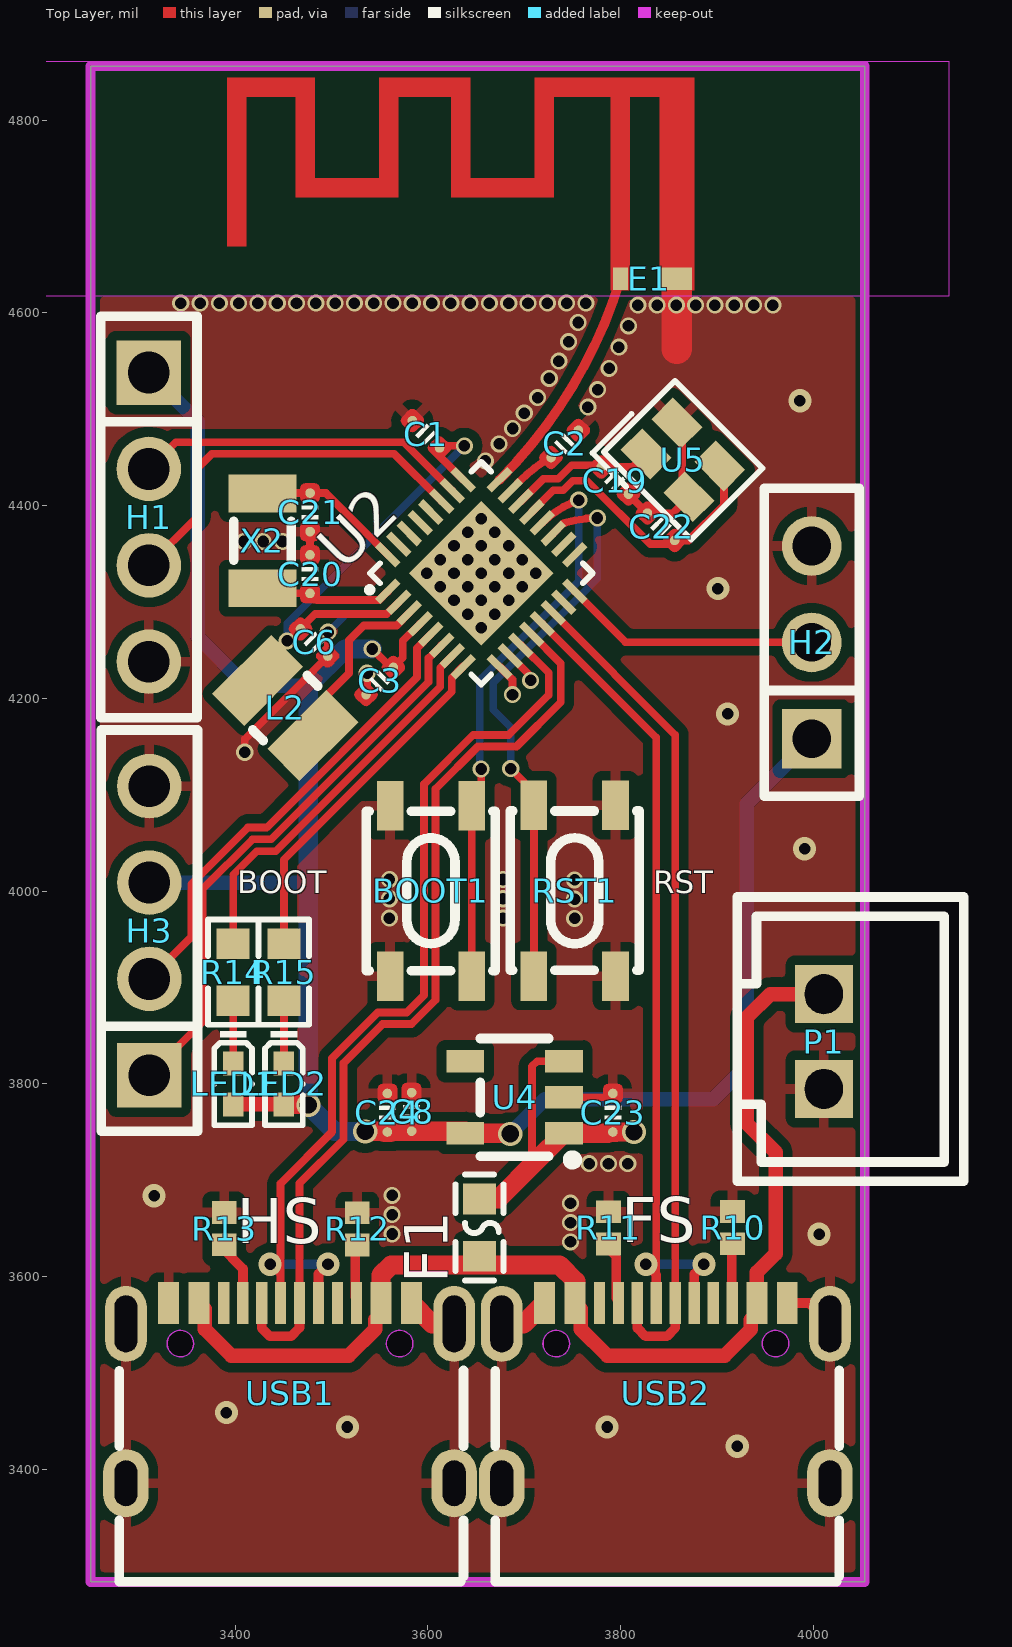
[diagram p0: Top Layer view]
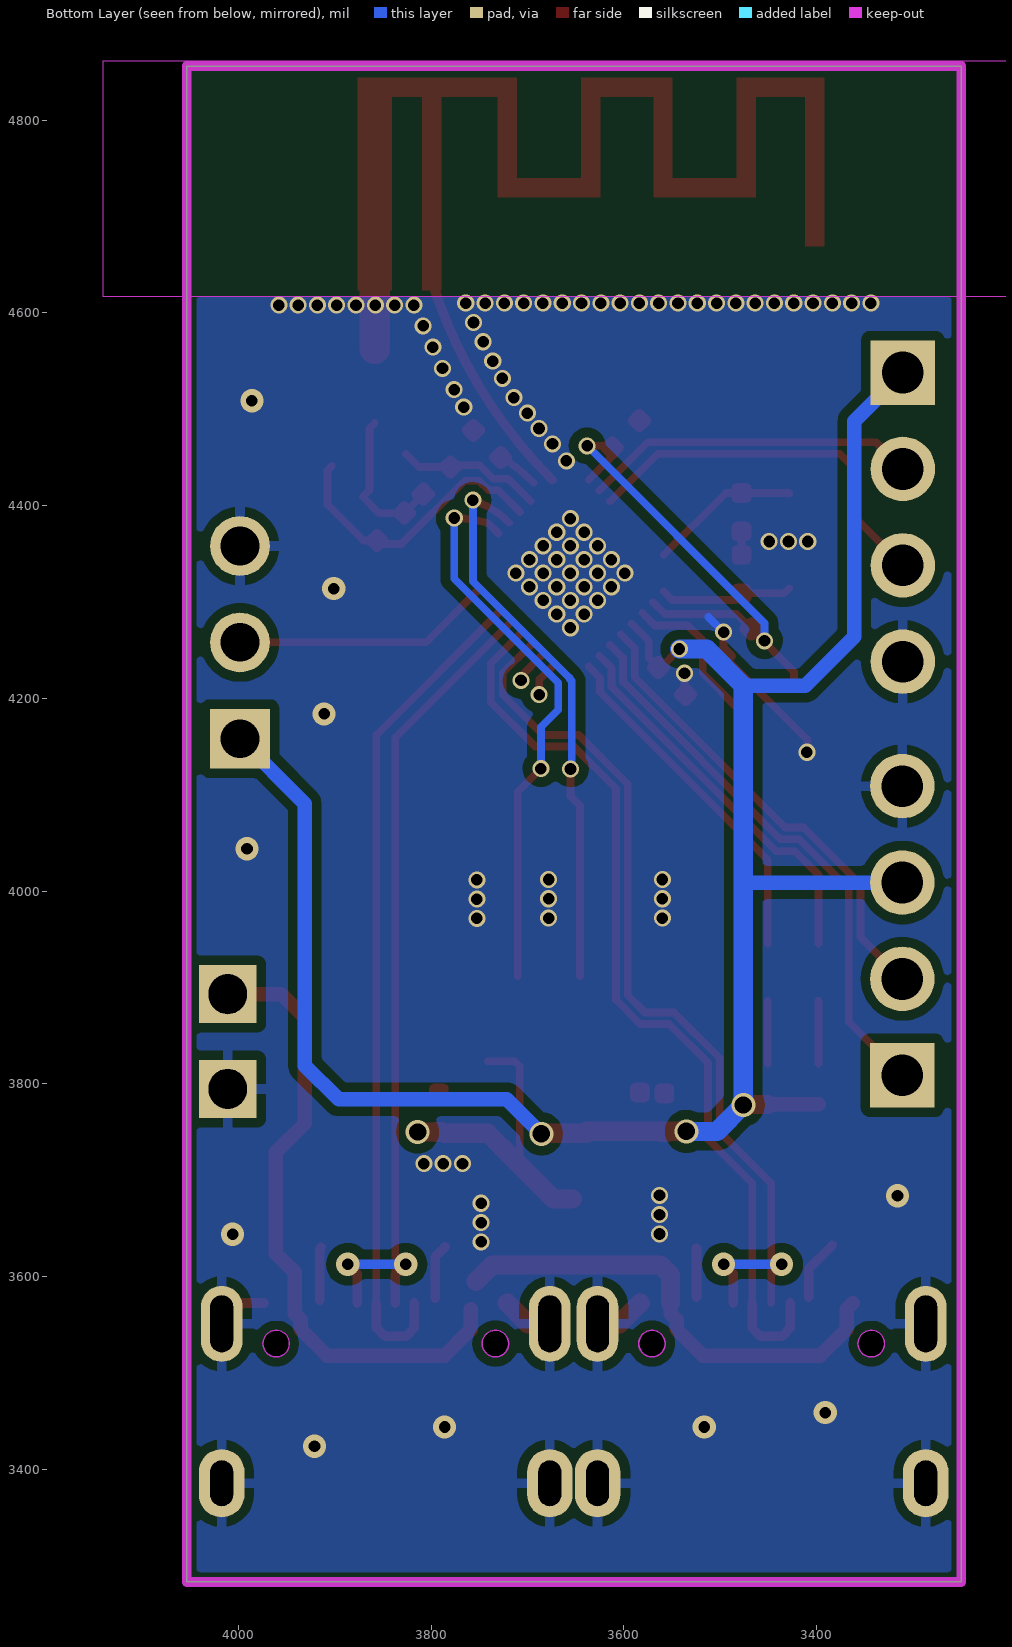
[diagram p1: Bottom Layer view, seen from below]
# Altium PCB MISC75430.pcbdoc
Units mil, origin at the board's own origin, x right, y up, seen from the top; angles counter-clockwise.
Board outline 803.38 x 1573.11 mil, 2 copper layers (Top Layer, Bottom Layer), stack 62.206 mil thick; 34 components, 40 nets, 141 pads, 120 vias.

## Layer stack, top to bottom
Top Solder Mask Layer: solder mask 0.394, Dk 3.3
Top Layer: signal copper 1.379
SUBSTRATE1: surface 59.449, FR4, Dk 4.5
Bottom Layer: signal copper 1.378
Bottom Solder Mask Layer: solder mask 0.394, Dk 3.3

## Board outline
3250,4856.14 3250,3283.03 4053.38,3283.03 4053.38,4856.14

## Design rules (kind name [scope] priority, off if disabled: settings)
BoardOutlineClearance copperThickness2oz_1 [All] p2 off: genericclearance=7.99 ignorepadtopadclearanceinfootprint=FALSE except(0: Arc-SplitContinuation Track-SplitContinuation SMDPad-SplitContinuation THPad-SplitContinuation Via-SplitContinuation Fill-SplitContinuation Region-SplitContinuation Poly-SplitContinuation Text-SplitContinuation Hole-SplitContinuation; 5.98: Arc-CutoutEdge Track-CutoutEdge SMDPad-CutoutEdge THPad-CutoutEdge Via-CutoutEdge Text-CutoutEdge; 6.9: Hole-OutlineEdge Hole-CutoutEdge; 10: Poly-OutlineEdge Poly-CutoutEdge; 11.81: Arc-OutlineEdge Track-OutlineEdge SMDPad-OutlineEdge THPad-OutlineEdge Via-OutlineEdge Fill-OutlineEdge Region-OutlineEdge Text-OutlineEdge Fill-CutoutEdge Region-CutoutEdge)
BoardOutlineClearance Plane_innerPlane_1 [All] p4 off: genericclearance=4.02 ignorepadtopadclearanceinfootprint=FALSE except(0: Arc-SplitContinuation Track-SplitContinuation SMDPad-SplitContinuation THPad-SplitContinuation Via-SplitContinuation Fill-SplitContinuation Region-SplitContinuation Poly-SplitContinuation Text-SplitContinuation Hole-SplitContinuation; 5.98: Arc-CutoutEdge Track-CutoutEdge SMDPad-CutoutEdge THPad-CutoutEdge Via-CutoutEdge Text-CutoutEdge; 6.9: Hole-OutlineEdge Hole-CutoutEdge; 10: Poly-OutlineEdge Poly-CutoutEdge; 11.81: Arc-OutlineEdge Track-OutlineEdge SMDPad-OutlineEdge THPad-OutlineEdge Via-OutlineEdge Fill-OutlineEdge Region-OutlineEdge Text-OutlineEdge Fill-CutoutEdge Region-CutoutEdge)
BoardOutlineClearance Copper_copperRegion_1 [All] p6 off: genericclearance=4.02 ignorepadtopadclearanceinfootprint=FALSE except(0: Arc-SplitContinuation Track-SplitContinuation SMDPad-SplitContinuation THPad-SplitContinuation Via-SplitContinuation Fill-SplitContinuation Region-SplitContinuation Poly-SplitContinuation Text-SplitContinuation Hole-SplitContinuation; 5.98: Arc-CutoutEdge Track-CutoutEdge SMDPad-CutoutEdge THPad-CutoutEdge Via-CutoutEdge Text-CutoutEdge; 6.9: Hole-OutlineEdge Hole-CutoutEdge; 10: Poly-OutlineEdge Poly-CutoutEdge; 11.81: Arc-OutlineEdge Track-OutlineEdge SMDPad-OutlineEdge THPad-OutlineEdge Via-OutlineEdge Fill-OutlineEdge Region-OutlineEdge Text-OutlineEdge Fill-CutoutEdge Region-CutoutEdge)
BoardOutlineClearance copperThickness1oz_1 [All] p8: genericclearance=0 ignorepadtopadclearanceinfootprint=FALSE except(0: Arc-OutlineEdge Track-OutlineEdge SMDPad-OutlineEdge THPad-OutlineEdge Via-OutlineEdge Fill-OutlineEdge Region-OutlineEdge Poly-OutlineEdge Text-OutlineEdge Hole-OutlineEdge Arc-CutoutEdge Track-CutoutEdge SMDPad-CutoutEdge THPad-CutoutEdge Via-CutoutEdge Fill-CutoutEdge Region-CutoutEdge Poly-CutoutEdge Text-CutoutEdge Hole-CutoutEdge Arc-SplitContinuation Track-SplitContinuation SMDPad-SplitContinuation THPad-SplitContinuation Via-SplitContinuation Fill-SplitContinuation Region-SplitContinuation Poly-SplitContinuation Text-SplitContinuation Hole-SplitContinuation)
Clearance copperThickness2oz [All] p1 off: gap=7.99 ignorepadtopadclearanceinfootprint=FALSE except(5.98: SMDPad-Track SMDPad-SMDPad THPad-Track SMDPad-THPad THPad-THPad Track-Via SMDPad-Via THPad-Via Via-Via Fill-SMDPad Region-SMDPad Fill-THPad Region-THPad Fill-Via Region-Via Fill-Fill Fill-Region Region-Region Arc-Track Arc-SMDPad Arc-THPad Arc-Via Fill-Arc Region-Arc Arc-Arc Text-Track SMDPad-Text Text-THPad Text-Via Fill-Text Region-Text Arc-Text Text-Text; 6.9: Hole-Track Hole-SMDPad Hole-THPad Hole-Via Fill-Hole Region-Hole Hole-Arc Hole-Text; 10: Poly-Track Poly-SMDPad Poly-THPad Poly-Via Poly-Fill Poly-Region Poly-Poly Poly-Arc Poly-Text Poly-Hole; 11.81: Fill-Track Region-Track)
Clearance Plane_innerPlane [All] p3 off: gap=4.02 ignorepadtopadclearanceinfootprint=FALSE except(5.98: SMDPad-Track SMDPad-SMDPad THPad-Track SMDPad-THPad THPad-THPad Track-Via SMDPad-Via THPad-Via Via-Via Fill-SMDPad Region-SMDPad Fill-THPad Region-THPad Fill-Via Region-Via Fill-Fill Fill-Region Region-Region Arc-Track Arc-SMDPad Arc-THPad Arc-Via Fill-Arc Region-Arc Arc-Arc Text-Track SMDPad-Text Text-THPad Text-Via Fill-Text Region-Text Arc-Text Text-Text; 6.9: Hole-Track Hole-SMDPad Hole-THPad Hole-Via Fill-Hole Region-Hole Hole-Arc Hole-Text; 10: Poly-Track Poly-SMDPad Poly-THPad Poly-Via Poly-Fill Poly-Region Poly-Poly Poly-Arc Poly-Text Poly-Hole; 11.81: Fill-Track Region-Track)
Clearance Copper_copperRegion [All] p5 off: gap=4.02 ignorepadtopadclearanceinfootprint=FALSE except(5.98: SMDPad-Track SMDPad-SMDPad THPad-Track SMDPad-THPad THPad-THPad Track-Via SMDPad-Via THPad-Via Via-Via Fill-SMDPad Region-SMDPad Fill-THPad Region-THPad Fill-Via Region-Via Fill-Fill Fill-Region Region-Region Arc-Track Arc-SMDPad Arc-THPad Arc-Via Fill-Arc Region-Arc Arc-Arc Text-Track SMDPad-Text Text-THPad Text-Via Fill-Text Region-Text Arc-Text Text-Text; 6.9: Hole-Track Hole-SMDPad Hole-THPad Hole-Via Fill-Hole Region-Hole Hole-Arc Hole-Text; 10: Poly-Track Poly-SMDPad Poly-THPad Poly-Via Poly-Fill Poly-Region Poly-Poly Poly-Arc Poly-Text Poly-Hole; 11.81: Fill-Track Region-Track)
Clearance copperThickness1oz [All] p7: gap=0 ignorepadtopadclearanceinfootprint=FALSE
DiffPairsRouting differentialPair [All] p1: maxlimit=6 minlimit=6 mostfreqgap=6 toplayer_minwidth=5 toplayer_prefwidth=10 toplayer_maxwidth=100 toplayer_mingap=6 toplayer_prefgap=6 toplayer_maxgap=6 bottomlayer_minwidth=5 bottomlayer_prefwidth=10 bottomlayer_maxwidth=100 bottomlayer_mingap=6 bottomlayer_prefgap=6 bottomlayer_maxgap=6 maxuncoupledlength=10
HoleToHoleClearance otherClearance [All] p1: gap=0 allowstackedmicrovias=TRUE
Length netLength [All] p1: minlimit=0 maxlimit=0
MatchedLengths netLengthTolerance [All] p1: tolerance=1000
PasteMaskExpansion pasteMaskExpansion [All] p1: expansion=0
PlaneConnect innerPlane [All] p1: planeconnectstyle=Relief reliefexpansion=20 reliefentries=4 reliefconductorwidth=10 reliefairgap=10
PolygonConnect copperRegion [All] p1: connectstyle=Relief reliefconductorwidth=10 reliefentries=4 polygonreliefangle="90 Angle" airgapwidth=10 via.connectstyle=Relief via.reliefconductorwidth=10 via.reliefentries=4 via.polygonreliefangle="90 Angle" via.airgapwidth=10
RoutingVias viaSize [All] p1: holewidth=0.39 width=0.39 viastyle="Through Hole" minholewidth=0.39 minwidth=0.39 maxholewidth=472.44 maxwidth=472.44
SolderMaskExpansion solderMaskExpansion [IsVia] p1: expansion=-1000 istentingtop=TRUE
SolderMaskExpansion solderMaskExpansion [All] p2: expansion=2 istentingtop=FALSE
Width copperThickness2oz_2 [All] p1 off: maxlimit=10 minlimit=10 preferedwidth=10 toplayer_minwidth=8 toplayer_maxwidth=100 toplayer_prefwidth=10 bottomlayer_minwidth=8 bottomlayer_maxwidth=100 bottomlayer_prefwidth=10
Width copperThickness1oz_2 [All] p2: maxlimit=10 minlimit=10 preferedwidth=10 toplayer_minwidth=5 toplayer_maxwidth=100 toplayer_prefwidth=10 bottomlayer_minwidth=5 bottomlayer_maxwidth=100 bottomlayer_prefwidth=10

## Components (designator, comment, footprint, x,y, rotation, side; value= is the part's Value field where it differs from the comment)
BOOT1 "K2-1808SN-A3SW-01" SW-SMD_4P-L4.2-W3.3-P2.15-LS5.1 3603.12,4000.1 r270 top
C1 "100nF" 0402电容（极简封装） 3598,4474 r135 top
C2 "470nF" 0402电容（极简封装） 3742,4464 r45 top
C3 "2.2uF" 0402电容（极简封装） 3550,4218 r225 top
C6 "4.7uF" 0402电容（极简封装） 3482,4258 r135 top
C8 "100nF" 0402电容（极简封装） 3583.17,3770.84 r270 top
C19 "NC" 0402电容（极简封装） 3794,4426 r135 top
C20 "NC" 0402电容（极简封装） 3477.72,4328.89 r90 top
C21 "NC" 0402电容（极简封装） 3477.81,4392.99 r270 top
C22 "NC" 0402电容（极简封装） 3842,4378 r315 top
C23 "1uF" 0402电容（极简封装） 3792,3770 r270 top
C24 "1uF" 0402电容（极简封装） 3558,3770 r270 top
E1 "" ANT-F-1-2.4G-1.6mmFR4 3662.08,4744.9 r0 top
F1 "BSMD0603-050-6V" F0603 3653.63,3650.83 r90 top
H1 "" HDR-TH_4P-P2.54-V-F 3310.5,4388.05 r270 top
H2 "" HDR-TH_3P-P2.54-V-F 3998.3,4258.05 r90 top
H3 "" HDR-TH_4P-P2.54-V-F 3311,3958.85 r90 top
L2 "10uH" IND-SMD_L2.5-W2.0 3452,4190 r135 top
LED1 "SZYY0402B" LED0402-RD_BLUE 3397.95,3799.79 r270 top
LED2 "SZYY0402B" LED0402-RD_BLUE 3450.63,3799.79 r270 top
P1 "XH2.54 through-hole socket-2P" CONN-TH_XH2.54-2P 4011,3843.85 r270 top
R10 "5.1kΩ" R0402 3916.19,3650.84 r270 top
R11 "5.1kΩ" R0402 3787.44,3650.56 r270 top
R12 "5.1kΩ" R0402 3526.84,3649.44 r270 top
R13 "5.1kΩ" R0402 3388.65,3649.68 r270 top
R14 "1kΩ" R0603 3397.95,3915.83 r270 top
R15 "1kΩ" R0603 3450.63,3915.83 r270 top
RST1 "K2-1808SN-A3SW-01" SW-SMD_4P-L4.2-W3.3-P2.15-LS5.1 3752.41,4000.34 r90 top
U2 "CH584F" QFN-32_L4.0-W4.0-P0.40-TL-EP2.7 3655.44,4329.85 r45 top
U4 "RT9013-33GB" SOT-23-5_L3.0-W1.7-P0.95-LS2.8-BR 3690,3786 r0 top
U5 "32MHz" CRYSTAL-SMD_4P-L2.0-W1.6-BL-2 3864.68,4447.36 r315 top
USB1 "TYPE-C 16PIN 2MD(073)" USB-C-SMD_TYPE-C-6PIN-2MD-073 3457,3479 r0 top
USB2 "TYPE-C 16PIN 2MD(073)" USB-C-SMD_TYPE-C-6PIN-2MD-073 3847,3479 r0 top
X2 "32.768kHz" FC-135R_L3.2-W1.5 3428.4,4363.43 r90 top

## Footprints (in the part's own frame and the unit in brackets; to place one, negate y for a bottom-side part, rotate by r counter-clockwise, add the part's x,y. Pads: shape width x height; smd on the part's side, far side on the other; paste and mask are expansions set on the pad)
0402电容（极简封装） [mil]
  round 10 smd: 1(-20,0) 2(20,0)
  Top Layer region: 30,-5 29.62,-6.91 28.54,-8.54 26.91,-9.62 25,-10 15,-10 13.09,-9.62 11.46,-8.54 10.38,-6.91 10,-5 10,5 10.38,6.91 11.46,8.54 13.09,9.62 15,10 25,10 26.91,9.62 28.54,8.54 29.62,6.91 30,5 30,-5
  Top Layer region: -10,-5 -10.38,-6.91 -11.46,-8.54 -13.09,-9.62 -15,-10 -25,-10 -26.91,-9.62 -28.54,-8.54 -29.62,-6.91 -30,-5 -30,5 -29.62,6.91 -28.54,8.54 -26.91,9.62 -25,10 -15,10 -13.09,9.62 -11.46,8.54 -10.38,6.91 -10,5 -10,-5
  silkscreen extent -7,-9 7,9
ANT-F-1-2.4G-1.6mmFR4 [mm]
  rect 0.8x0.6 smd paste+0 mask+0: 0(4.984,-2.785)
  rect 0.4x0.6 smd paste+0 mask+0: 1(3.501,-2.785)
  Top Layer region: 3.741,-3.089 3.741,2.243 3.241,2.243 3.241,-3.089
  Top Layer region: 5.441,-3.089 5.441,2.217 4.541,2.217 4.541,-3.089
  Top Layer region: 5.441,2.012 5.441,2.512 1.241,2.512 1.241,2.012
  Top Layer region: 1.741,-0.628 1.741,2.192 1.241,2.192 1.241,-0.628
  Top Layer region: 1.651,-0.628 1.651,-0.134 -0.889,-0.134 -0.889,-0.628
  Top Layer region: -0.459,-0.628 -0.459,2.192 -0.959,2.192 -0.959,-0.628
  Top Layer region: -0.459,2.012 -0.459,2.512 -2.859,2.512 -2.859,2.012
  Top Layer region: -2.359,-0.628 -2.359,2.192 -2.859,2.192 -2.859,-0.628
  Top Layer region: -2.374,-0.628 -2.374,-0.128 -4.863,-0.128 -4.863,-0.628
  Top Layer region: -4.559,-0.628 -4.559,2.192 -5.059,2.192 -5.059,-0.628
  Top Layer region: -4.559,2.012 -4.559,2.512 -6.859,2.512 -6.859,2.012
  Top Layer region: -6.359,-1.928 -6.359,2.192 -6.859,2.192 -6.859,-1.928
CONN-TH_XH2.54-2P [mil]
  rect 60x60 hole 39.37 slot 41.34 at 0 deg paste+0 mask+1.97: 1(-49.21,0) 2(49.21,0)
  silkscreen extent -150,-90 145,145
CRYSTAL-SMD_4P-L2.0-W1.6-BL-2 [mm]
  rect 1.1x0.8 smd: 1(-0.8,-0.575) 2(0.8,-0.575) 3(0.8,0.575) 4(-0.8,0.575)
  silkscreen extent -1.82,-1.56 1.64,1.33
F0603 [mil]
  rect 31.75x34.02 smd paste-3937.01 mask+2: 1(-29.66,0) 2(29.66,0)
  silkscreen extent -55,-25 55,25
FC-135R_L3.2-W1.5 [mm]
  rect 1x1.8 smd: 1(-1.25,0) 2(1.25,0)
  silkscreen extent -0.51,-0.76 0.51,0.76
HDR-TH_3P-P2.54-V-F [mil]
  rect 62x62 hole 40.16: 1(-100,0)
  round 62 hole 40.16: 2(0,0) 3(100,0)
  silkscreen extent -160,-49 160,49
HDR-TH_4P-P2.54-V-F [mm]
  rect 1.7x1.7 hole 1.1: 1(-3.81,0)
  round 1.7 hole 1.1: 2(-1.27,0) 3(1.27,0) 4(3.81,0)
  silkscreen extent -5.29,-1.27 5.29,1.27
IND-SMD_L2.5-W2.0 [mm]
  rect 1.2x2.2 smd: 1(1.028,0) 2(-1.028,0)
  silkscreen extent -0.2,-1.02 0.2,1.02
LED0402-RD_BLUE [mm]
  rect 0.636x0.54 smd paste-100 mask+0.051: 1(-0.538,0) 2(0.538,0)
  silkscreen extent -1.39,-0.54 1.09,0.54
QFN-32_L4.0-W4.0-P0.40-TL-EP2.7 [mm]
  rect 0.76x0.2 smd paste-100 mask+0.051: 1(-2.08,1.4) 2(-2.08,1) 3(-2.08,0.6) 4(-2.08,0.2) 5(-2.08,-0.2) 6(-2.08,-0.6) 7(-2.08,-1) 8(-2.08,-1.4) 17(2.08,-1.4) 18(2.08,-1) 19(2.08,-0.6) 20(2.08,-0.2) 21(2.08,0.2) 22(2.08,0.6) 23(2.08,1) 24(2.08,1.4)
  rect 0.2x0.76 smd paste-100 mask+0.051: 9(-1.4,-2.08) 10(-1,-2.08) 11(-0.6,-2.08) 12(-0.2,-2.08) 13(0.2,-2.08) 14(0.6,-2.08) 15(1,-2.08) 16(1.4,-2.08) 25(1.4,2.08) 26(1,2.08) 27(0.6,2.08) 28(0.2,2.08) 29(-0.2,2.08) 30(-0.6,2.08) 31(-1,2.08) 32(-1.4,2.08)
  rect 2.7x2.7 smd paste-100 mask+0.051: 33(0,0)
  silkscreen extent -2.46,-2.08 2.08,2.08
R0402 [mm]
  rect 0.6x0.65 smd paste+0 mask+0.051: 1(-0.425,0) 2(0.425,0)
R0603 [mil]
  rect 31.75x34.02 smd paste-3937.01 mask+2: 1(-29.66,0) 2(29.66,0)
  silkscreen extent -55,-26 55,26
SOT-23-5_L3.0-W1.7-P0.95-LS2.8-BR [mm]
  rect 1x0.6 smd paste+0 mask+0.051: 1(1.3,-0.95) 2(1.3,0) 3(1.3,0.95) 4(-1.3,0.95) 5(-1.3,-0.95)
  silkscreen extent -0.9,-1.78 1.65,1.55
SW-SMD_4P-L4.2-W3.3-P2.15-LS5.1 [mm]
  rect 1.3x0.7 smd: 1(-2.25,1.075) 2(2.25,1.075) 3(-2.25,-1.075) 4(2.25,-1.075)
  silkscreen extent -2.1,-1.7 2.1,1.7
USB-C-SMD_TYPE-C-6PIN-2MD-073 [mm]
  rect 0.55x1.1 smd paste-100 mask+0.05: 1(-3.2,2.375) 2(-2.4,2.375) 11(2.4,2.375) 12(3.2,2.375)
  rect 0.3x1.1 smd paste-100 mask+0.05: 3(-1.75,2.375) 4(-1.25,2.375) 5(-0.75,2.375) 6(-0.25,2.375) 7(0.25,2.375) 8(0.75,2.375) 9(1.25,2.375) 10(1.75,2.375)
  oval 1.2x1.8 hole 0.6 slot 1.2 at 90 deg paste+0 mask+0.05: 13(-4.325,-2.375) 14(4.325,-2.375)
  oval 1.1x2 hole 0.6 slot 1.5 at 90 deg paste+0 mask+0.05: 13(-4.325,1.825) 14(4.325,1.825)
  Board Outline Layer circle w0.003: c-2.89,1.305 r0.35
  Board Outline Layer circle w0.003: c2.89,1.305 r0.35
  Board Outline Layer region: -2.54,1.305 -2.575,1.153 -2.672,1.031 -2.812,0.964 -2.968,0.964 -3.108,1.031 -3.205,1.153 -3.24,1.305 -3.24,1.305 -3.205,1.457 -3.108,1.579 -2.968,1.646 -2.812,1.646 -2.672,1.579 -2.575,1.457 -2.54,1.305
  Board Outline Layer region: -2.54,1.305 -2.549,1.227 -2.575,1.153 -2.616,1.087 -2.672,1.031 -2.738,0.99 -2.812,0.964 -2.89,0.955 -2.968,0.964 -3.042,0.99 -3.108,1.031 -3.164,1.087 -3.205,1.153 -3.231,1.227 -3.24,1.305 -3.231,1.383 -3.205,1.457 -3.164,1.523 -3.108,1.579 -3.042,1.62 -2.968,1.646 -2.89,1.655 -2.812,1.646 -2.738,1.62 -2.672,1.579 -2.616,1.523 -2.575,1.457 -2.549,1.383
  Board Outline Layer region: 3.24,1.305 3.205,1.153 3.108,1.031 2.968,0.964 2.812,0.964 2.672,1.031 2.575,1.153 2.54,1.305 2.54,1.305 2.575,1.457 2.672,1.579 2.812,1.646 2.968,1.646 3.108,1.579 3.205,1.457 3.24,1.305
  Board Outline Layer region: 3.24,1.305 3.231,1.227 3.205,1.153 3.164,1.087 3.108,1.031 3.042,0.99 2.968,0.964 2.89,0.955 2.812,0.964 2.738,0.99 2.672,1.031 2.616,1.087 2.575,1.153 2.549,1.227 2.54,1.305 2.549,1.383 2.575,1.457 2.616,1.523 2.672,1.579 2.738,1.62 2.812,1.646 2.89,1.655 2.968,1.646 3.042,1.62 3.108,1.579 3.164,1.523 3.205,1.457 3.231,1.383
  Multi-Layer board cut-out: -2.54,1.305 -2.575,1.153 -2.672,1.031 -2.812,0.964 -2.968,0.964 -3.108,1.031 -3.205,1.153 -3.24,1.305 -3.24,1.305 -3.205,1.457 -3.108,1.579 -2.968,1.646 -2.812,1.646 -2.672,1.579 -2.575,1.457 -2.54,1.305
  Multi-Layer board cut-out: 3.24,1.305 3.205,1.153 3.108,1.031 2.968,0.964 2.812,0.964 2.672,1.031 2.575,1.153 2.54,1.305 2.54,1.305 2.575,1.457 2.672,1.579 2.812,1.646 2.968,1.646 3.108,1.579 3.205,1.457 3.24,1.305
  silkscreen extent -4.5,-4.97 4.57,0.6

## Via types
v1: diameter 17.72, hole 12, Top Layer to Bottom Layer, 102 vias
v2: diameter 24.02, hole 12, Top Layer to Bottom Layer, 14 vias
v3: diameter 25, hole 18, Top Layer to Bottom Layer, 4 vias

## Nets (pads, with @x,y where several pads share a name; then routed paths per layer and width w, separated by ;. In a path a pad name is that pad's centre, name@x,y a point inside that pad or via, vN(x,y) a via of type N, cw(c..) or ccw(c..) an arc to the next point about the centre after c; other vN are vias at no path point)
$1N6708: R10.2 USB2.10 | length 55.7
  Top Layer w10: R10.2@3913.82,3630.41 3915.39,3628.84 USB2.10@3915.39,3575.38
$1N6711: R11.2 USB2.4 | length 57.3
  Top Layer w10: R11.2@3785.53,3630.72 3795.59,3620.66 USB2.4@3795.59,3577.58
$1N6713: R12.2 USB1.10 | length 50.9
  Top Layer w10: USB1.10@3524.59,3578.79 3524.59,3629.1 R12.2@3525.01,3629.52
$1N6715: R13.2 USB1.4 | length 63.9
  Top Layer w10: R13.2@3383.67,3632.45 3408.19,3607.93 USB1.4@3408.19,3578.68
$1N6755: LED1.1 R14.2 | length 65.2
  Top Layer w8: LED1.1 R14.2
$1N6756: LED2.1 R15.2 | length 65.2
  Top Layer w8: LED2.1 R15.2
+5V: C23.2 F1.2 U4.1 U4.3 | length 318.3
  Top Layer w8: 3712.89,3720.3 3708,3725.2 3708,3818 3713.4,3823.4 U4.3
  Top Layer w20: F1.2 3673.07,3680.49 3712.89,3720.3 U4.1 3786.6,3748.6 ; C23.2 v3(3814,3750)
ANT: E1.1 U2.24 | length 245.8
  Top Layer w10: U2.24 ccw(c3317.35,4783.75) E1.1
BOOT: BOOT1.1 BOOT1.2 U2.20 | length 586
  Top Layer w8: BOOT1.2 BOOT1.1 3655.32,4098.56 v1(3655.32,4126.68) ; U2.20 cw(c3787.84,4313.26) v1(3756.61,4405.61)
  Bottom Layer w8: v1(3655.32,4126.68) 3654,4128 3654,4218 3655.98,4219.98 3655.98,4220.98 3756.61,4321.6 v1(3756.61,4405.61)
GND: BOOT1.3 BOOT1.4 C1.2 C2.2 C3.2 C6.1 C8.1 C19.1 C20.2 C21.2 C22.1 C23.1 C24.1 E1.0 H1.4 H2.3 H3.4 P1.2 R10.1 R11.1 R12.1 R13.1 RST1.3 RST1.4 U2.33 U4.2 U5.2 U5.4 USB1.1 USB1.12 USB1.13 USB1.14 USB2.1 USB2.12 USB2.13 USB2.14 | length 674.2
  Top Layer w8: v1(3410,4144) 3410,4157.72 C6.1 3496.49,4244.21 v1(3496.49,4268.73) ; C20.2 3477.81,4348.97 C21.2 ; C3.2 3537.04,4205.04 v1(3537.04,4226) ; U4.2 3788,3786 C23.1 ; C19.1 C22.1 3854,4392.14 U5.2 3864,4416.04 3864,4480.05 U5.4
  Top Layer w10: USB2.12 3995.62,3572.51 USB2.14@4017.28,3550.86
  Top Layer w20: USB1.12 3604.64,3550.86 USB1.14@3627.28,3550.86 ; USB2.13@3676.72,3550.86 3699.36,3550.86 USB2.1
  Top Layer w31.5: 3858.3,4562.41 E1.0
  Bottom Layer w8: v1(3496.49,4268.73) 3512.08,4284.32
  other v1: 3748,3635.98 3562.99,3644.16 3748,3656 3562.99,3664.18 3748,3676.02 3562.99,3684.19 3767.42,3717.17 3787.44,3717.17 3807.46,3717.17 3560,3971.98 3678,3971.98 3752.4,3971.58 3560,3992 3678,3992 3752.4,3991.6 3560,4012.02 3678,4012.02 3752.4,4011.62 3655.44,4273.23 3641.28,4287.39 3669.59,4287.39 3627.13,4301.54 3655.44,4301.54 3683.74,4301.54 3612.97,4315.7 3641.28,4315.7 3669.59,4315.7 3697.9,4315.7 3598.82,4329.85 3627.13,4329.85 3655.44,4329.85 3683.74,4329.85 3712.05,4329.85 3612.97,4344.01 3641.28,4344.01 3669.59,4344.01 3697.9,4344.01 3627.13,4358.16 3655.44,4358.16 3683.74,4358.16 3409.12,4362.7 3429.14,4362.7 3449.15,4362.7 3641.28,4372.32 3669.59,4372.32 3655.44,4386.47 3659.67,4446.36 3674,4464 3688,4480 3700,4496 3766.07,4502.18 3714,4512 3776.11,4520.25 3726,4532 3788.16,4542.33 3736,4550 3798.2,4564.42 3746,4570 3808.24,4586.51 3756,4590 3817.86,4608 3837.87,4608 3857.89,4608 3877.91,4608 3897.93,4608 3917.95,4608 3937.96,4608 3957.98,4608 3343.62,4610 3363.64,4610 3383.66,4610 3403.68,4610 3423.69,4610 3443.71,4610 3463.73,4610 3483.75,4610 3503.77,4610 3523.78,4610 3543.8,4610 3563.82,4610 3583.84,4610 3603.86,4610 3623.87,4610 3643.89,4610 3663.91,4610 3683.93,4610 3703.95,4610 3723.96,4610 3743.98,4610 3764,4610
  other v2: 3921,3423.85 3516.58,3443.85 3786,3443.85 3391,3458.85 4006,3643.85 3316,3683.85 3991,4043.85 3911,4183.85 3901,4313.85 3986,4508.85
PA4: H1.2 U2.26 | length 347.2
  Top Layer w8: H1.2 3338.31,4465.86 3575.1,4465.86 U2.26
PA5: H1.3 U2.27 | length 401.6
  Top Layer w8: H1.3 3361,4388.55 3361,4438.85 3376,4453.85 3564.85,4453.85 U2.27
PA10: C20.1 U2.1 X2.1 | length 138.9
  Top Layer w8: X2.1 3433.73,4308.89 C20.1 3484.61,4302 3549.63,4302 U2.1
PA11: C21.1 U2.32 X2.2 | length 156.9
  Top Layer w8: X2.2 3428.76,4412.99 C21.1 3494.35,4412.99 U2.32
PA12: U2.31
PA13: U2.30
PA14: U2.29
PA15: U2.28
PB4: U2.18
PB5: U2.17
PB6: H2.2 U2.16 | length 267.9
  Top Layer w8: U2.16 3805.19,4258.05 H2.2
PB7: U2.15
PB8: H3.1 U2.6 | length 583.4
  Top Layer w8: H3.1 3366.46,3864.31 3366.46,4002.2 3418.11,4053.85 3437.61,4053.85 3600.77,4217 3600.77,4241.78 U2.6
PB9: H3.2 U2.5 | length 490
  Top Layer w8: H3.2 3354.45,3952.29 3354.45,4007.17 3413.14,4065.86 3432.64,4065.86 3588.75,4221.98 3588.75,4252.04 U2.5
PB10: U2.14 USB2.5 USB2.7 | length 866.9
  Top Layer w8: U2.14 3856.84,4161.85 USB2.7
  Top Layer w10: USB2.5 3817.47,3546.53 3826,3538 3848,3538 3856.84,3546.84 USB2.7
PB11: U2.13 USB2.6 USB2.8 | length 873.7
  Top Layer w8: U2.13 3837.16,4159.26 3837.16,3601.83
  Top Layer w10: v2(3826.31,3612.68) 3837.16,3601.83 USB2.6 ; USB2.8 3876.53,3602.78 v2(3886.42,3612.68)
  Bottom Layer w10: v2(3826.31,3612.68) v2(3886.42,3612.68)
PB12: U2.12 USB1.5 USB1.7 | length 957.9
  Top Layer w8: USB1.7 3466.84,3696.84 3512.58,3742.58 3512.58,3821.59 3552.98,3861.98 3582.98,3861.98 3608.02,3887.02 3608.02,4106.02 3652,4150 3692,4150 3738,4196 3738,4236.16 U2.12
  Top Layer w10: USB1.5 3427.47,3546.53 3436,3538 3458,3538 3466.84,3546.84 USB1.7
PB13: U2.11 USB1.6 USB1.8 | length 969
  Top Layer w8: v2(3436.31,3612.68) 3447.16,3601.83 ; USB1.6 3447.16,3601.83 ; U2.11 3725.54,4226.34 3725.54,4203.54 3684,4162 3647.01,4162 3596,4110.99 3596,3892 3578,3874 3548,3874 3500.56,3826.56 3500.56,3749.94 3447.16,3696.53 3447.16,3601.83
  Top Layer w10: USB1.8 3486.53,3602.78 v2(3496.42,3612.68)
  Bottom Layer w10: v2(3436.31,3612.68) v2(3496.42,3612.68)
PB14: U2.10 | length 34.3
  Top Layer w8: U2.10 3706.67,4222.94 v1(3706.67,4218.57)
PB15: U2.9 | length 34.7
  Top Layer w8: U2.9 3687.86,4219.48 v1(3687.86,4203.86)
PB16: R15.1 U2.8 | length 364.5
  Top Layer w8: R15.1 3450.63,4032.63 3624.8,4206.8 3624.8,4221.27 U2.8
PB17: R14.1 U2.7 | length 404.2
  Top Layer w8: R14.1 3398,4016.74 3422.53,4041.27 3442.03,4041.27 3612.78,4212.02 3612.78,4231.52 U2.7
PB23: RST1.1 RST1.2 U2.19 | length 587.9
  Top Layer w8: v1(3686,4127.11) 3710.09,4103.02 RST1.2 RST1.1 ; U2.19@3730.03,4371.04 3740.61,4381.61 3741.63,4381.61 ; 3742,4382 cw(c3775.93,4271.43) v1(3775.93,4387.09)
  Bottom Layer w8: v1(3686,4127.11) 3686,4170 3668,4188 3668,4216 3775.93,4323.93 v1(3775.93,4387.09)
VCC: C3.1 C8.2 C24.2 H1.1 H2.1 H3.3 LED1.2 LED2.2 U2.4 U4.5 | length 2141.3
  Top Layer w8: v1(3542.32,4251.16) 3561.33,4232.14 C3.1 3574,4242 3574,4259.55 U2.4
  Top Layer w15: LED1.2 LED2.2
  Top Layer w20: LED2.2 3475.4,3778.6 v3(3476,3778) ; v3(3535.06,3750.6) 3535.3,3750.84 C8.2 U4.5@3638.82,3750.84 ; U4.5 3684.92,3748.6 v3(3685.52,3748)
  Bottom Layer w15: H1.1 3361,4487.55 3361,4263.85 3411.72,4213.12 3476,4213.12 ; H3.3 3476,4008.85 ; v3(3685.52,3748) 3721.36,3783.85 3896,3783.85 3931,3818.85 3931,4090.75 H2.1
  Bottom Layer w20: v3(3535.06,3750.6) 3503.4,3750.6 v3(3476,3778) 3476,4008.85 3476,4213.12 3514.03,4251.16 v1(3542.32,4251.16)
VDCIA: C1.1 C6.2 L2.1 U2.2 U2.25 | length 533.7
  Top Layer w8: L2.1 3423.38,4227.66 C6.2 3483.29,4287.58 3557.48,4287.58 U2.2 ; U2.25 3612.14,4451.1 C1.1 3614.28,4462 v1(3638,4462)
  Bottom Layer w8: v1(3454,4259.69) 3454,4278 v1(3638,4462)
VIN: F1.1 P1.1 USB1.2 USB1.11 USB2.2 USB2.11 | length 1157.9
  Top Layer w15: USB1.2 3368.72,3566.3 3368.72,3545.27 3395.98,3518 3518.03,3518 3545.29,3545.27 3545.29,3555.29 3551.49,3561.49 USB1.11 ; USB2.2@3758.72,3566.3 3758.72,3545.27 3785.98,3518 3908.03,3518 3935.29,3545.27 3935.29,3555.29 3941.49,3561.49 USB2.11 3941.49,3604.34 3961,3623.85 3961,3728.85 3931,3758.85 3931,3868.85 3955.22,3893.06 P1.1
  Top Layer w20: USB1.11 3551.49,3601.49 3562,3612 3736.61,3612 3753.41,3595.2
VINTA: C2.1 U2.23 | length 35
  Top Layer w8: U2.23@3693.5,4423.6 cw(c3824.47,4292.63) 3720.48,4445.9
VSW: L2.2 U2.3 | length 188.8
  Top Layer w8: L2.2 3480.62,4188.45 3518.2,4226.02 3518.2,4260.2 3533.56,4275.56 3567.74,4275.56 U2.3
X32MI: C19.2 U2.22 U5.1 | length 149.9
  Top Layer w8: U2.22 3719.98,4427.8 3734.06,4427.8 3734.23,4427.97 3735.33,4427.97 3749.36,4442 C19.2@3777.12,4442 ; C19.2@3779.42,4439.7 C19.2@3780.65,4438.48 ; C19.2 3812.92,4440.14 U5.1
X32MO: C22.2 U2.21 U5.3 | length 300.8
  Top Layer w8: U2.21 3730.24,4415.79 3739.04,4415.79 3739.21,4415.95 3740.3,4415.95 3750.23,4425.88 3764.99,4425.88 3830.77,4360.09 C22.2@3859.12,4360.09 ; C22.2 3870.46,4363.86 3907.38,4400.78 3907.38,4436.68 U5.3
pads on no net: U4.4 USB1.3 USB1.9 USB2.3 USB2.9

## Polygon pours and split planes (outlines as drawn)
GND on Bottom Layer (solid, remove dead copper, pour order 2): 3136,4952 3136,3240 4414,3240 4414,4952
GND on Top Layer (solid, remove dead copper, pour order 0): 3000,5002 3000,3000 4108,3000 4108,5002

## Keep-outs
Board Outline Layer:
  region: 4140.48,4617 3158.29,4617 3158.29,4861.18 4140.49,4861.18
  lines w10: 3250,3283.03 3250,4856.14 4053.38,4856.14 4053.38,3283.03 3250,3283.03

## Silkscreen, mask and mechanical layers (free items; w line width, h text height)
Top Silkscreen Layer:
  text "BOOT" at 3402,3990 h40
  text "RST" at 3834,3990 h40
  text "FS" at 3800.57,3620.24 h80
  text "HS" at 3401.95,3619.01 h80